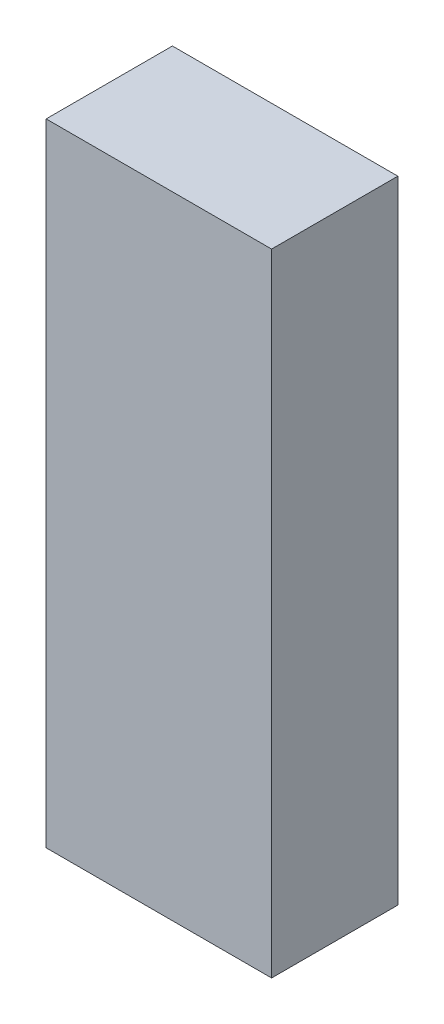
from build123d import *

# Parameters (mm, degrees)
SKETCH_1_W      = 25
SKETCH_1_H      = 70
EXTRUDE_1_DEPTH = 7


with BuildPart() as part:
    # 草图1 → 凸台-拉伸1 (new, symmetric)
    with BuildSketch(Plane.XY):
        Rectangle(SKETCH_1_W, SKETCH_1_H)
    extrude(amount=EXTRUDE_1_DEPTH, both=True)


solid = part.part
